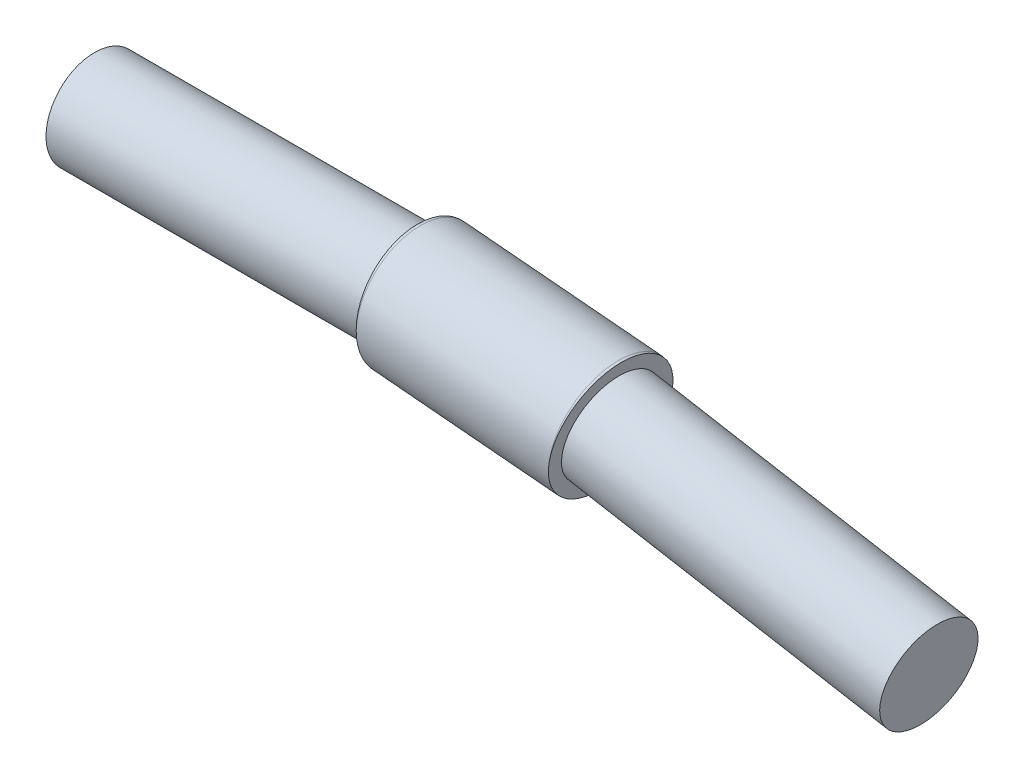
SolidWorks part; units mm, degrees
ref_plane "前视基准面" through (0, 0, 0) normal (0, 0, 1) x (1, 0, 0)
ref_plane "上视基准面" through (0, 0, 0) normal (0, 1, 0) x (1, 0, 0)
ref_plane "右视基准面" through (0, 0, 0) normal (1, 0, 0) x (0, 0, -1)
sketch "草图1" plane through (0, 0, 0) normal (0, 0, 1) x (1, 0, 0)
  line L0 (0, 0) -> (50, 0)
  line L1 (50, 0) -> (79.8858, -2.6147)
  line L2 (79.8858, -2.6147) -> (129.1262, -11.2971)
  dimension "D1" = 50
  dimension "D2" = 30
  dimension "D3" = 50
  dimension "D4" = 175
  dimension "D5" = 175
sketch "草图2" plane through (0, 0, 0) normal (1, 0, 0) x (0, 0, -1)
  circle A0 centre (0, 0) radius 9.5
  dimension "D1" = 19
sweep "扫描1" add profiles "草图2" path "草图1"
sketch "草图3" plane through (0, 0, 0) normal (-1, 0, 0) x (0, 0, 1)
  circle A0 centre (0, 0) radius 7.5
  dimension "D1" = 15
extrude "切除-拉伸1" cut sketch "草图3" against normal blind 50 flip side to cut
cosmetic thread "装饰螺纹线1" parameters "D1"=30, "D2"=11.797
sketch "草图4" plane through (127.1645, -22.4225, 0) normal (0.9848, -0.1736, 0) x (0, 0, -1)
  circle A0 centre (0, 11.2971) radius 7.5
  dimension "D1" = 15
extrude "切除-拉伸2" cut sketch "草图4" against normal blind 50 flip side to cut
cosmetic thread "装饰螺纹线2" parameters "D1"=30, "D2"=11.797
ref_plane "基准面1" through (1.2078, 13.8051, 0) normal (0.0872, 0.9962, 0) x (0.9962, -0.0872, 0)
sketch "草图7" plane through (1.2078, 13.8051, 0) normal (0.0872, 0.9962, 0) x (0.9962, -0.0872, 0)
  line L0 (64.8097, 9.5) -> (64.8097, -9.5) construction
  line L1 (79.8097, 9.5) -> (49.8097, 9.5) construction
  line L2 (49.8097, -9.5) -> (79.8097, -9.5) construction
ref_plane "基准面3" through (64.5631, -5.6485, 0) normal (-0.9962, 0.0872, 0) x (0, 0, 1)
